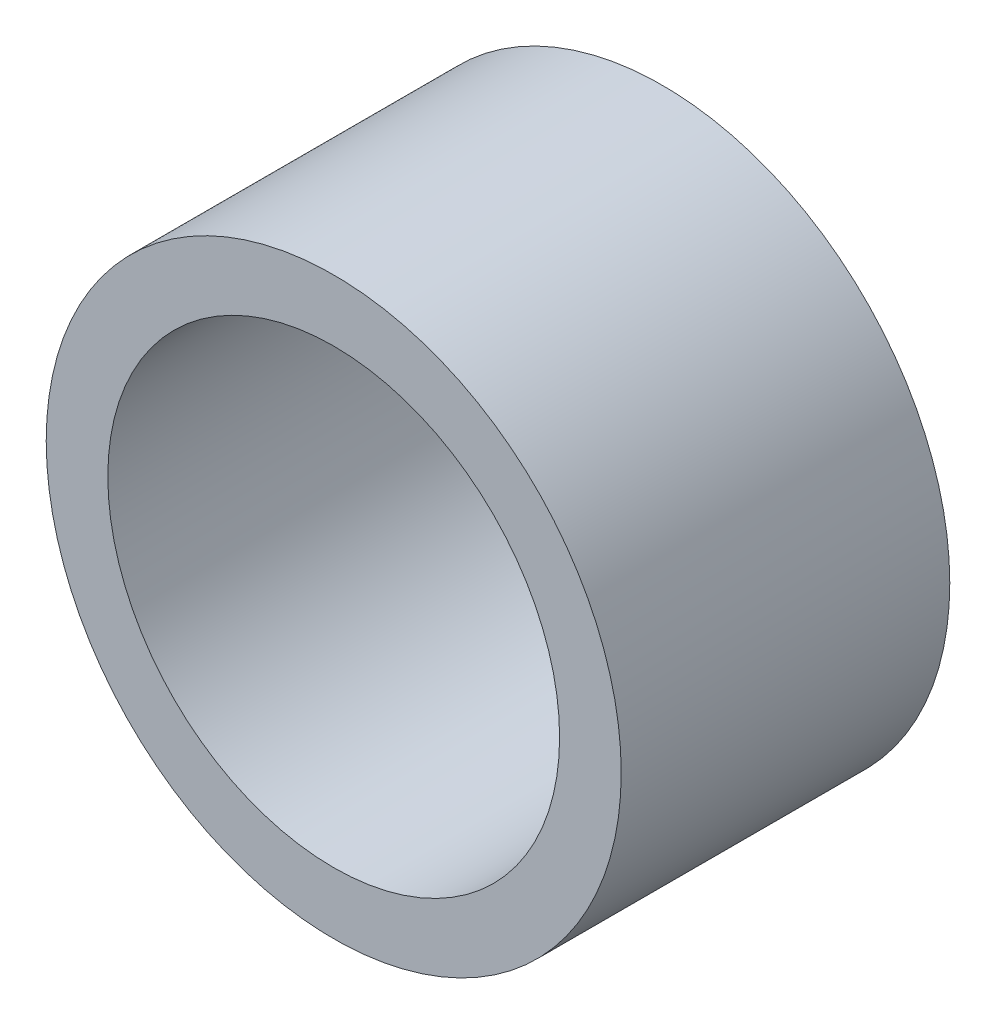
SolidWorks part; units mm, degrees
ref_plane "前视基准面" through (0, 0, 0) normal (0, 0, 1) x (1, 0, 0)
ref_plane "上视基准面" through (0, 0, 0) normal (0, 1, 0) x (1, 0, 0)
ref_plane "右视基准面" through (0, 0, 0) normal (1, 0, 0) x (0, 0, -1)
other "Configuration Table"
sketch "草图1" plane through (0, 0, 0) normal (0, 0, 1) x (1, 0, 0)
  circle A0 centre (0, 0) radius 35
  circle A1 centre (0, 0) radius 27.5
  dimension "D1" = 55
  dimension "D2" = 70
extrude "凸台-拉伸1" add sketch "草图1" along normal blind 40
